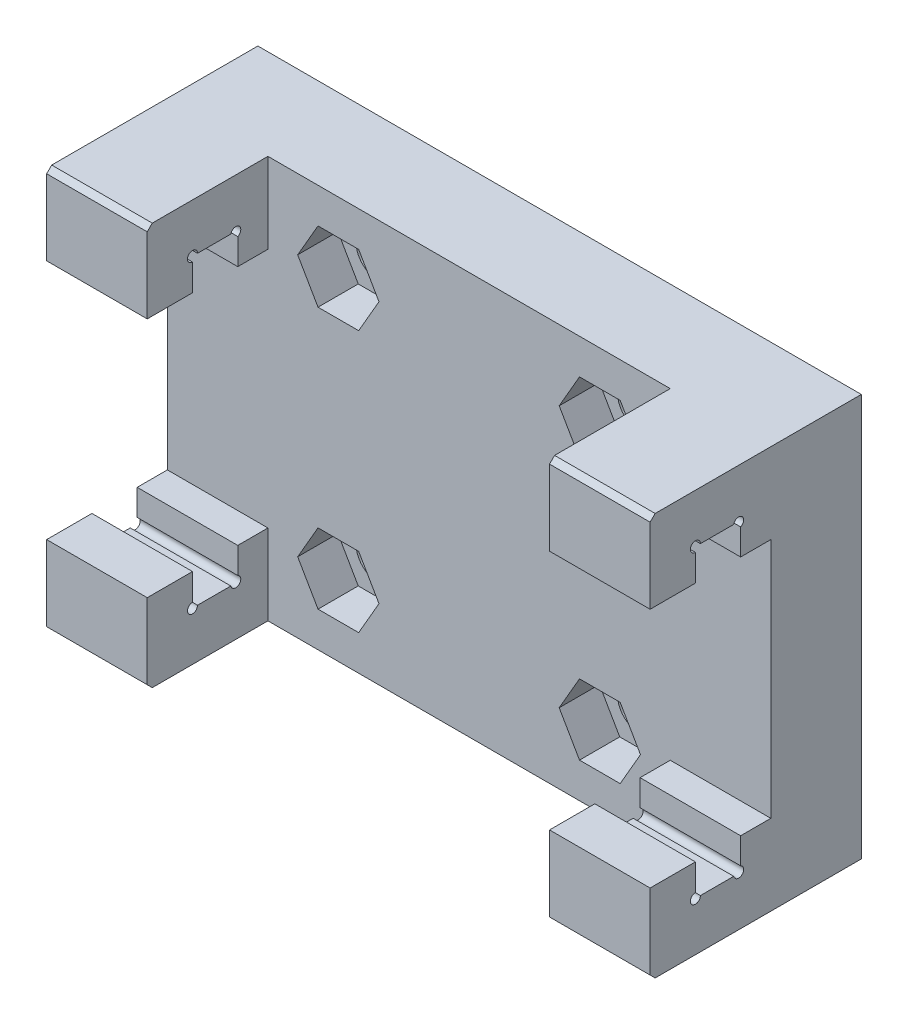
from build123d import *

# Parameters (mm, degrees)
SKETCH_1_W               = 60
SKETCH_1_H               = 40
EXTRUDE_1_DEPTH          = 21
SKETCH_2_W               = 40
SKETCH_2_H               = 46.112845628
CUT_EXTRUDE_1_DEPTH      = 12
SKETCH_3_W               = 80.513519028
SKETCH_3_H               = 24
CUT_EXTRUDE_2_DEPTH      = 12
SKETCH_4_W               = 4.5
SKETCH_4_H               = 30.3
CUT_EXTRUDE_3_DEPTH      = 67.640828326
SKETCH_5_R               = 2.25
CUT_EXTRUDE_4_DEPTH      = 12
MIRROR_2_COPY_1_SKETCH_R = 2.25
MIRROR_2_COPY_1_DEPTH    = 12
CUT_EXTRUDE_5_DEPTH      = 4
MIRROR_4_COPY_1_DEPTH    = 4
SKETCH_7_R               = 0.5
CUT_EXTRUDE_6_DEPTH      = 67.640828326
CHAMFER_1_SIZE           = 0.5


with BuildPart() as part:
    # 草图1 → 凸台-拉伸1 (new body)
    with BuildSketch(Plane.XY):
        Rectangle(SKETCH_1_W, SKETCH_1_H)
    extrude(amount=EXTRUDE_1_DEPTH)

    # 草图2 → 切除-拉伸1 (cut)
    with BuildSketch(Plane.XY.offset(21)):
        Rectangle(SKETCH_2_W, SKETCH_2_H)
    extrude(amount=-CUT_EXTRUDE_1_DEPTH, mode=Mode.SUBTRACT)

    # 草图3 → 切除-拉伸2 (cut)
    with BuildSketch(Plane.XY.offset(21)):
        Rectangle(SKETCH_3_W, SKETCH_3_H)
    extrude(amount=-CUT_EXTRUDE_2_DEPTH, mode=Mode.SUBTRACT)

    # 草图4 → 切除-拉伸3 (cut, through all)
    with BuildSketch(Plane.ZY.offset(30)):
        with Locations((14.25, 0)):
            Rectangle(SKETCH_4_W, SKETCH_4_H)
    extrude(amount=-CUT_EXTRUDE_3_DEPTH, mode=Mode.SUBTRACT)

    # 草图5 → 切除-拉伸4 (cut)
    with BuildSketch(Plane.XY.offset(9)):
        with Locations((-13, 13)):
            Circle(SKETCH_5_R)
    cut_extrude_4 = extrude(amount=-CUT_EXTRUDE_4_DEPTH, mode=Mode.SUBTRACT)

    # 镜向1: 切除-拉伸4 across plane
    add(cut_extrude_4.mirror(Plane.ZX), mode=Mode.SUBTRACT)

    # 镜向2: 切除-拉伸4 across plane
    add(cut_extrude_4.mirror(Plane(origin=(0, 0, 0), x_dir=(0, 0, 1), z_dir=(1, 0, 0))), mode=Mode.SUBTRACT)

    # 镜向2 copy 1 sketch → 镜向2 copy 1 (cut)
    with BuildSketch(Plane(origin=(0, 0, 9), x_dir=(-1, 0, 0), z_dir=(0, 0, 1))):
        with Locations((-13, 13)):
            Circle(MIRROR_2_COPY_1_SKETCH_R)
    extrude(amount=-MIRROR_2_COPY_1_DEPTH, mode=Mode.SUBTRACT)

    # 草图6 → 切除-拉伸5 (cut)
    with BuildSketch(Plane.XY.offset(9)):
        Polygon((-8.958548116, 13), (-10.979274058, 16.5), (-15.020725942, 16.5), (-17.041451884, 13), (-15.020725942, 9.5), (-10.979274058, 9.5), align=None)
    cut_extrude_5 = extrude(amount=-CUT_EXTRUDE_5_DEPTH, mode=Mode.SUBTRACT)

    # 镜向3: 切除-拉伸5 across plane
    add(cut_extrude_5.mirror(Plane(origin=(0, 0, 0), x_dir=(0, 0, 1), z_dir=(1, 0, 0))), mode=Mode.SUBTRACT)

    # 镜向4: 切除-拉伸5 across plane
    add(cut_extrude_5.mirror(Plane.ZX), mode=Mode.SUBTRACT)

    # 镜向4 copy 1 sketch → 镜向4 copy 1 (cut)
    with BuildSketch(Plane(origin=(0, 0, 9), x_dir=(-1, 0, 0), z_dir=(0, 0, 1))):
        Polygon((-8.958548116, 13), (-10.979274058, 16.5), (-15.020725942, 16.5), (-17.041451884, 13), (-15.020725942, 9.5), (-10.979274058, 9.5), align=None)
    extrude(amount=-MIRROR_4_COPY_1_DEPTH, mode=Mode.SUBTRACT)

    # 草图7 → 切除-拉伸6 (cut, through all)
    with BuildSketch(Plane.ZY.offset(30)):
        with Locations((12.2, 15.05)):
            Circle(SKETCH_7_R)
        with Locations((16.5, 15.15)):
            Circle(SKETCH_7_R)
    cut_extrude_6 = extrude(amount=-CUT_EXTRUDE_6_DEPTH, mode=Mode.SUBTRACT)

    # 镜向5: 切除-拉伸6 across plane
    add(cut_extrude_6.mirror(Plane.ZX), mode=Mode.SUBTRACT)

    # 倒角1
    chamfer_1_edges = [part.edges().sort_by_distance(p)[0] for p in [
        (-25, 20, 21),
        (25, -20, 21),
        (-25, -20, 21),
        (25, 20, 21),
    ]]
    chamfer(chamfer_1_edges, length=CHAMFER_1_SIZE)


solid = part.part
